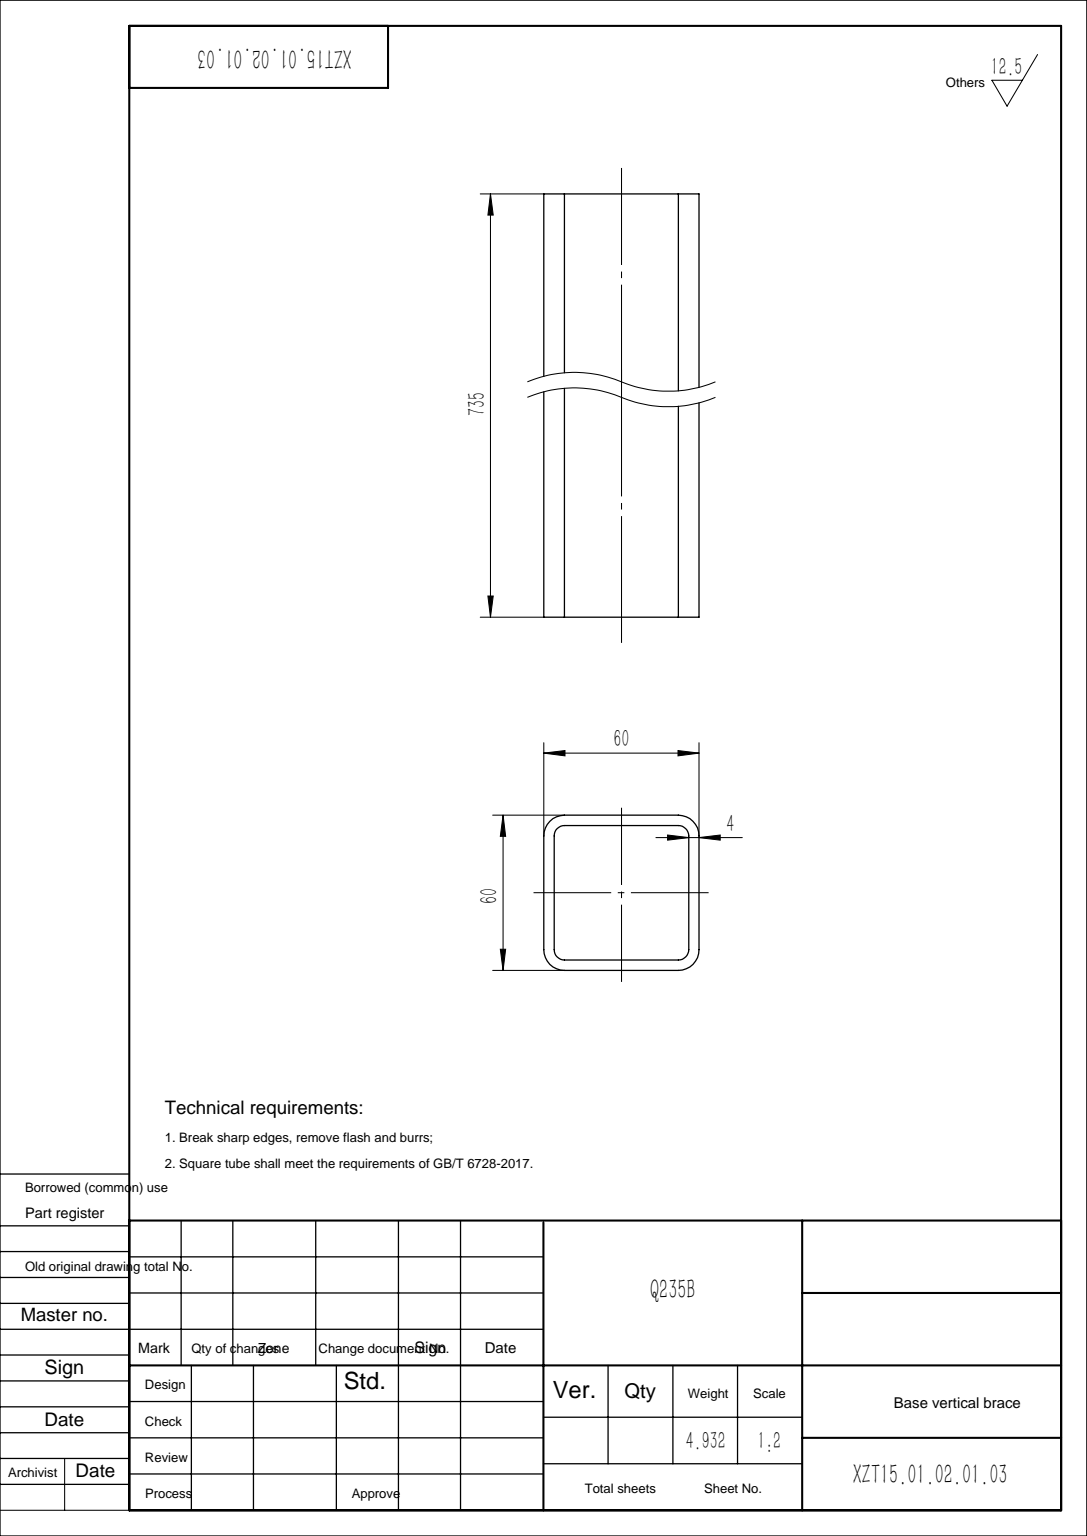
SolidWorks part; units mm, degrees
material "Q235B"
ref_plane "Front Plane" through (0, 0, 0) normal (0, 0, 1) x (1, 0, 0)
ref_plane "Top Plane" through (0, 0, 0) normal (0, 1, 0) x (1, 0, 0)
ref_plane "Right Plane" through (0, 0, 0) normal (1, 0, 0) x (0, 0, -1)
sketch "草图1" plane through (0, 0, 0) normal (0, 0, 1) x (1, 0, 0)
  line L0 (0, 0) -> (0, 735)
  dimension "D1" = 735
other "GB/T 6728-2002 square hollow section 60×60×4(1)"
ref_plane "Plane1" through (0, 0, 0) normal (0, 1, 0) x (-1, 0, 0)
sketch "Sketch1" plane through (0, 0, 0) normal (0, 1, 0) x (-1, 0, 0)
  line L0 (-22, -26) -> (22, -26)
  line L1 (-26, -22) -> (-26, 22)
  line L2 (22, 26) -> (-22, 26)
  line L3 (26, 22) -> (26, -22)
  line L4 (-22, -30) -> (22, -30)
  line L5 (-30, -22) -> (-30, 22)
  line L6 (22, 30) -> (-22, 30)
  line L7 (30, 22) -> (30, -22)
  arc A0 (30, 22) -> (22, 30) centre (22, 22) ccw
  arc A1 (22, -30) -> (30, -22) centre (22, -22) ccw
  arc A2 (-30, -22) -> (-22, -30) centre (-22, -22) ccw
  arc A3 (-22, 30) -> (-30, 22) centre (-22, 22) ccw
  arc A4 (-22, 26) -> (-26, 22) centre (-22, 22) ccw
  arc A5 (26, 22) -> (22, 26) centre (22, 22) ccw
  arc A6 (22, -26) -> (26, -22) centre (22, -22) ccw
  arc A7 (-26, -22) -> (-22, -26) centre (-22, -22) ccw
  point P0 (-30, 0)
  point P1 (30, 0)
  point P2 (0, 30)
  point P3 (0, -30)
  point P4 (0, 0)
  point P5 (-30, -30)
  point P6 (30, -30)
  point P7 (30, 30)
  point P8 (-30, 30)
  point P33 (0, 0)
  dimension "D1" = 8
  dimension "Thickness" = 4
  dimension "V_leg" = 60
